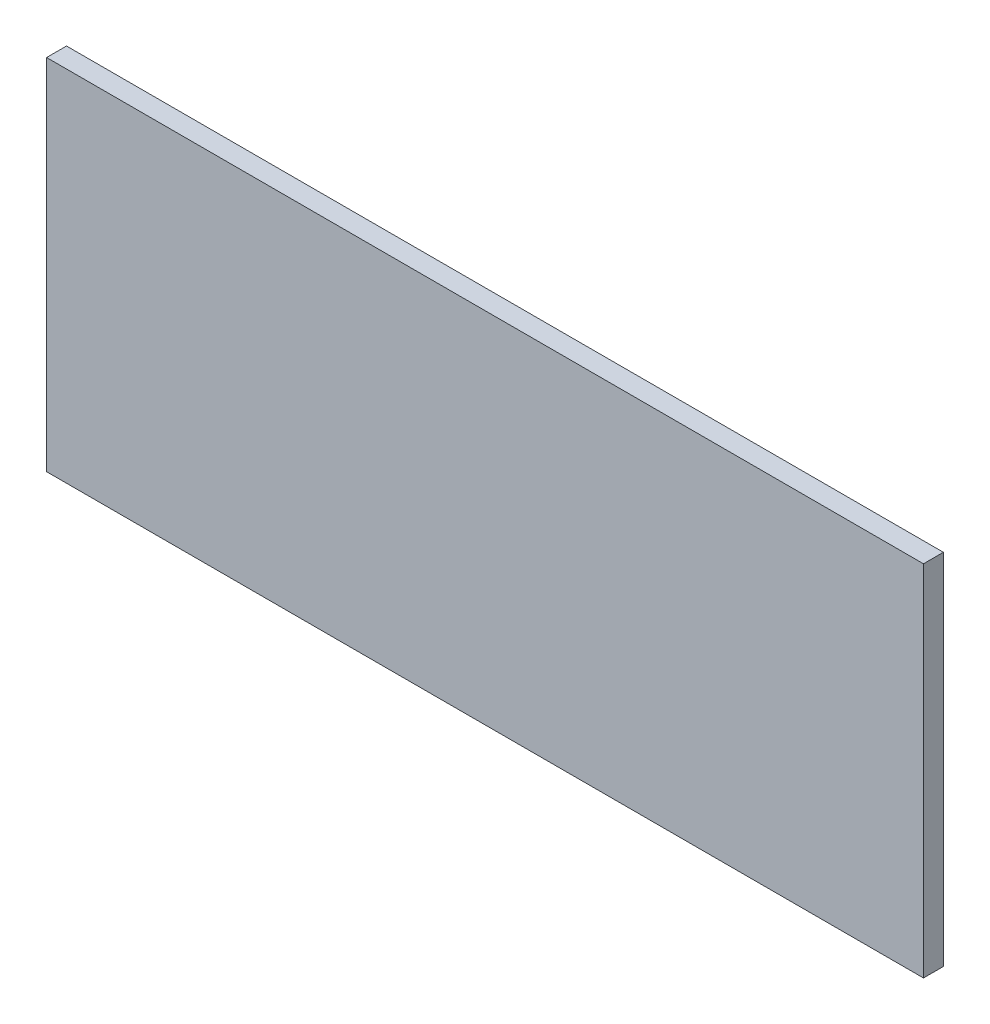
SolidWorks part; units mm, degrees
ref_plane "前视基准面" through (0, 0, 0) normal (0, 0, 1) x (1, 0, 0)
ref_plane "上视基准面" through (0, 0, 0) normal (0, 1, 0) x (1, 0, 0)
ref_plane "右视基准面" through (0, 0, 0) normal (1, 0, 0) x (0, 0, -1)
sketch "草图1" plane through (0, 0, 0) normal (0, 0, 1) x (1, 0, 0)
  line L0 (0, 0) -> (440, 0)
  line L1 (440, 0) -> (440, -180)
  line L2 (440, -180) -> (0, -180)
  line L3 (0, -180) -> (0, 0)
extrude "凸台-拉伸1" add sketch "草图1" along normal blind 10
sketch "草图2" plane through (0, 0, 10) normal (0, 0, 1) x (1, 0, 0)
  line L0 (220, -180) -> (220, 52.6961)
  line L1 (0, -180) -> (440, -180) construction
